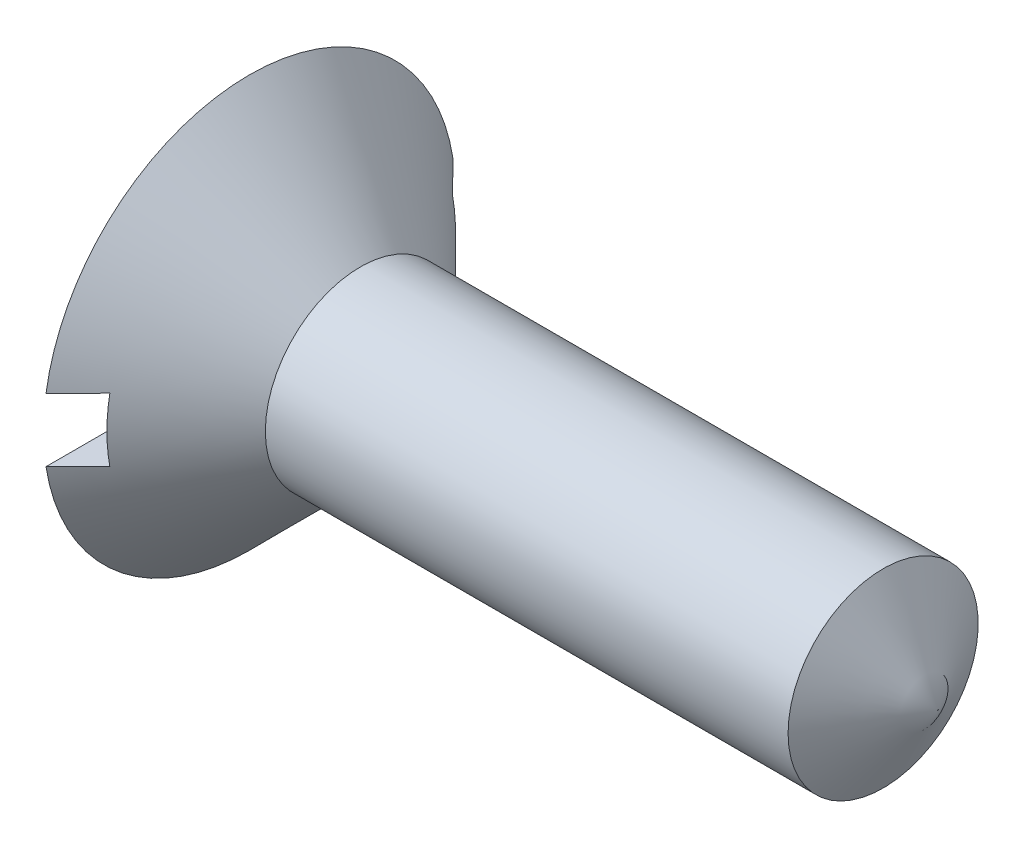
from build123d import *

# Parameters (mm, degrees)
CUT_EXTRUDE1_DEPTH      = 12
CUT_EXTRUDE1_DEPTH_BACK = 10
SKETCH2_W               = 2
SKETCH2_H               = 2


with BuildPart() as part:
    # Sketch1 → Revolve1 (revolve)
    with BuildSketch(Plane.XY, mode=Mode.PRIVATE) as revolve1_sk:
        Polygon((0, 0), (0, 6.5), (3.5, 3), (20, 3), (21.732050808, 0), align=None)
    revolve(revolve1_sk.sketch.rotate(Axis((0, 0, 0), (1, 0, 0)), 90), axis=Axis((0, 0, 0), (1, 0, 0)))

    # Sketch2 → Cut-Extrude1 (cut, two sides: drawn at the far end of the back side and taken through both)
    with BuildSketch(Plane.XY.offset(-CUT_EXTRUDE1_DEPTH_BACK)):
        Rectangle(SKETCH2_W, SKETCH2_H)
    extrude(amount=CUT_EXTRUDE1_DEPTH + CUT_EXTRUDE1_DEPTH_BACK, mode=Mode.SUBTRACT)


solid = part.part
